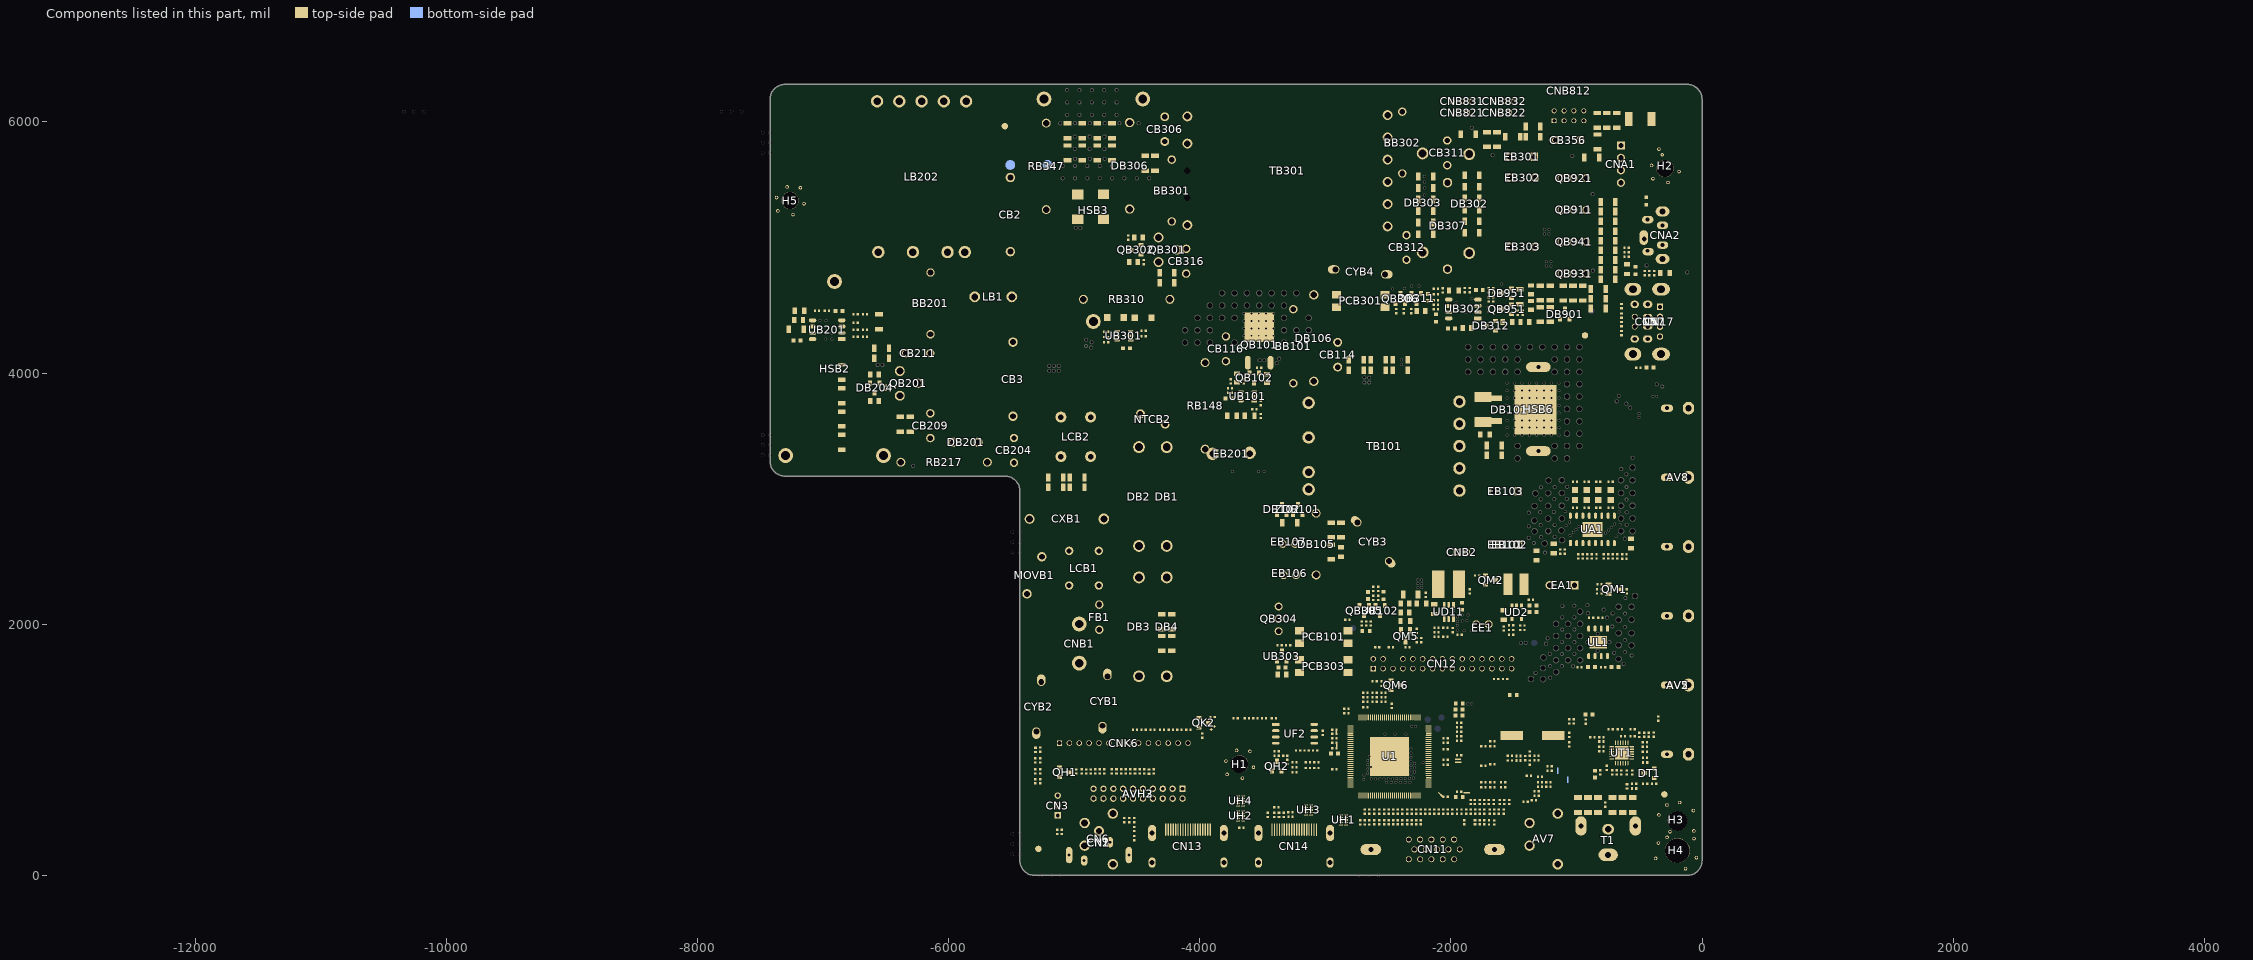
[diagram p0: the components of this part, seen from the top]
# Altium PCB MISC84277.PcbDoc (part 5 of 15)
Units mil, origin at the board's own origin, x right, y up, seen from the top; angles counter-clockwise.
Board outline 7422.08 x 6299.21 mil, 2 copper layers (TopLayer, BottomLayer), stack 61.855 mil thick; 709 components, 395 nets, 2812 pads, 811 vias.

## Footprints (in the part's own frame and the unit in brackets; to place one, negate y for a bottom-side part, rotate by r counter-clockwise, add the part's x,y. Pads: shape width x height; smd on the part's side, far side on the other; paste and mask are expansions set on the pad) (continued)
USB2-HD-1 [mm] "双盟 DUAL USB A/F 90°"
  oval 2.9x3.7 on Top Overlay: 0(-6.57,16) 0(-6.57,10.3) 0(6.57,16) 0(6.57,10.3)
  round 1.85 on Top Overlay: 0(-3.5,13.01) 0(-3.5,15.63) 0(3.5,13.01) 0(3.5,15.63)
  round 1.4 on Top Overlay: 0(-1,15.63) 0(-1,13.01) 0(1,15.63) 0(1,13.01)
  oval 1.5x1.7 hole 0.9: 1(-3.5,15.63) 4(3.5,15.63) 5(-3.5,13.01) 8(3.5,13.01)
  round 1.2 hole 0.9: 2(-1,15.63) 3(1,15.63) 6(-1,13.01) 7(1,13.01)
  oval 2.6x3.4 hole 1.6 slot 2.3 at 90 deg: 9(-6.57,16) 10(6.57,16) 11(-6.57,10.3) 12(6.57,10.3)
  KeepOutLayer pour cut-out: -5.206,13.033 -5.206,15.649 -4.578,15.021 -4.578,13.669 -5.214,13.033
  KeepOutLayer pour cut-out: -3.49,14.749 -4.146,14.618 -4.703,14.246 -5.075,13.69 -5.206,13.033 -5.206,13.033 -5.206,12.993 -5.068,12.303 -4.677,11.718 -4.092,11.327 -3.402,11.19 -3.402,11.19 2.42,11.19 2.637,11.233 2.821,11.356 2.943,11.539 2.986,11.756 2.986,11.756 2.986,14.202 2.944,14.414 2.824,14.594 2.644,14.714 2.432,14.756 2.432,14.756 -3.482,14.756 -3.485,14.756 -3.487,14.754 -3.489,14.752 -3.49,14.749
  KeepOutLayer pour cut-out: -3.49,17.369 -4.146,17.238 -4.703,16.866 -5.075,16.31 -5.206,15.653 -5.206,15.653 -5.206,15.613 -5.068,14.923 -4.677,14.338 -4.092,13.947 -3.402,13.81 -3.402,13.81 2.42,13.81 2.637,13.853 2.821,13.976 2.943,14.159 2.986,14.376 2.986,14.376 2.986,16.822 2.944,17.034 2.824,17.214 2.644,17.334 2.432,17.376 2.432,17.376 -3.482,17.376 -3.485,17.376 -3.487,17.374 -3.489,17.372 -3.49,17.369
  silkscreen extent -6.7,2 6.7,17.25, body extent -7.5,0 7.5,17, height 16.1
VR(13*5)-V-7.5 [mm] "TVR10561KSW(为勤)"
  round 1.9 hole 1.2: 1(3.75,-1.5) 2(-3.75,1.5)
  round 2.1 on Top Overlay: 2(-3.75,1.5) 2(3.75,-1.5)
  silkscreen extent -6.65,-2.5 6.42,2.5
XTAL-S-1 [mm] "假贴晶振（威特电子）"
  rect 4.6x1.8 smd: 1(-4.207,0) 2(4.207,0)
  silkscreen extent -5.8,-2.41 5.8,2.41, body extent -6.4,-2.36 6.39,2.38, height 5

## Part data
AV2 AV8: library part "RCA端子,RCA Jack,AV3,H,Yellow、White、Red,CH5.5,D14,Seal,DIP,RC075-F03L3BY-A,YUQIU-DLMI-AV", "CN-AV-D14-#-#"
AV5: library part "RCA端子,RCA Jack,AV3,H,Green、Blue、Red,CH5.5,D14,Seal,DIP,RC075-F03L3BY-B,YUQIU-DLMI-YPbPr", "CN-YPbPr-D14-#-#"
AV7: library part "耳机端子,Earphone  Jack,H,Φ3.5,CH7.0,Black,Seal,SMD,PJ7723-F03L3BE-C,YUQIU-DLMI", "CN-headphone"
AVH2: library part "连接插座,connect jack,2×10Pin,D2.0,D,SNAP,Fool-proofing,Beige,L=2.6mm,DIP,CJ-DHMI", "CN-latched"
AVH3: library part 2*10PIN-2.0-D-H-M-DHMI, "CN-straight gold pin"
BB101: library part φ3.5×6.0×0.65mm-CP(编带/秀益达)-9-DAI, "Through-hole ferrite bead"
BB201: library part Φ3.5×9.0×0.65mm(编带/秀益达)-DLAI, "Through-hole ferrite bead"
BB301: library part φ3.5×6.0×0.65mm-CP(编带/秀益达)-DAI, "Through-hole ferrite bead"
BB302: library part φ3.5×6.0×0.65mm-CP(编带/RY)-DLAI, "Through-hole ferrite bead"
C1: library part 10uF-1206-X5R-±10%-16V-D
CA9 CA10 CA16 CA17 CA24 CA25 CB103 CB323 CB324 CF29 CF30 CF33: library part 1000pF-0402-X7R-±10%-50V-D
CA11 CA23 CD2 CD3 CD6 CL2 CL3 CL42 CL43: library part 0.1uF-0402-X5R-±20%-16V-D
CA12 CA13 CA14 CA18 CA19 CA20 CA21 CA22: library part 0.22uF-0402-X5R-±10%-16V-D
CA15: library part 1uF-0402-X5R-±20%-16V-D
CA31 CA32 CD13: library part 3300pF-0402-X7R-±10%-50V-D
CA40 CA41 CD1 CD5 CD8 CD9 CD10 CM5: library part 10uF-0805-X5R-±20%-16V-D
CA60 CA61 CT12 CT19: library part 0.022uF-0402-X7R-±10%-16V-D
CB2 CB3: library part MPX450K474(散装/日精)-DHMI, "CAP(474)"
CB101 CB303 CB305 CI2 CO9 CT17: library part 100pF-0402-NPO-±5%-50V-D
CB102 CB109 CB206 CB304 CB321: library part 0.1uF-0603-X7R-±10%-50V-D, "CAP"
CB110 CB340: library part 1000pF-0402-X7R-±10%-50V-D, "CAP"
CB111 CB112: library part 1uF-0805-X7R-±10%-25V-D, "CAP"
CB113: library part 220PF-0805-NPO-±10%-200V-D, "CAP"
CB114 CB306: library part C242G472J20A201(编带/法拉)-DAI, "CAP"
CB116 CB209 CB316: library part "陶瓷电容,CAP CD,1KV,100pF,±10%,SL,P,5.0mm,DIP,TP,SHM-DHAI", "CAP"
CB118: library part 1000pF-0805-NPO-±10%-200V-D, "CAP"
CB201: library part 0.047uF-0603-X7R-±10%-25V-D
CB204: library part "陶瓷电容,CAP CD,1KV,4700pF,±20%,Y5U,P,5.0mm,DIP,TP,SHM-DHAI"
CB205: library part 220pF-0402-NPO-±5%-50V-D
CB211 CB312: library part CC45SL3AD470JYPNA(TDK)-DHAI, "CAP"
CB212: library part 0.22uF-0805-X7R-±10%-50V-D
CB221 CB301 CO10 CO11: library part 4700pF-0402-X7R-±10%-50V-D
CB302: library part "陶瓷电容,CAP MC,25V,1uF,±10%,X7R,0603,SMD,TP-D", "CAP"
CB311: library part "CAP CD,1KV,1000pF,±10%,Y5R,P,5.0mm,DIP,TP,SHM-DHAI", "CAP"
CB322: library part 0.022uF-0603-X7R-±10%-25V-D
CB326: library part 0.33uF-0805-X7R-±10%-50V-D, "C"
CB327 CB951: library part 0.1uF-0402-X7R-±10%-16V-D, "CAP"
CB328: library part 0.047uF-0805-X7R-±10%-50V-D
CB350: library part 0.47uF-0603-X5R-±10%-16V-D
CB356: library part CK45-B3AD102KYPNX(TDK)-DHAI, "CAP"
CD4 CD11 CD14 CD15 CF3 CF5 CF15 CF22 CF28 CF37 CL4 CL44 CT2 CT6 CU1: library part 10uF-0603-X5R-±20%-6.3V-D
CD7 CI8 CK6 CO8: library part 10pF-0402-NPO-±5%-50V-D
CD12 CD16 CD17 CF2 CF7 CF8 CF9 CF10 CF12 CF13 CF14 CF17 CF27 CG1 CG2 CH4 CH8 CH9 CH15 CI3 CI4 CI5 CI6 CK1 CK3 CK10 CM1 CM2 CM4 CO6 CT1 CT5 CT9 CT11 CT18 CT20 CT21 CT23 CT25 CT27 CT30 CV5 CV6: library part 0.1uF-0402-Y5V-+80%-20%-16V-D
CF1 CF32 CF38 CF39: library part 30pF-0402-NPO-±5%-50V-D
CF4 CH3 CH7 CH10 CT7 CT8 CV9 CV10: library part 33pF-0402-NPO-±5%-50V-D
CF6 CF11 CF16 CF18 CF19 CF20 CF21 CF23 CF24 CF25 CO1 CO4: library part 1uF-0402-X5R-±20%-6.3V-D
CF26 CF31 CF34 CI1 CI7 CI9 CI11 CV1 CV3 CV7: library part 0.047uF-0402-X7R-±10%-16V-D
CF35 CF36: library part 5pF-0402-NPO-±5%-50V-D
CK2 CM7: library part 0.01uF-0402-X7R-±10%-50V-D
CM3: library part 0.22uF-0402-Y5V-+80%-20%-16V-D
CN1: library part "RCA端子,RCA Jack,AV1,H,Yellow,CH5.5,Seal,DIP,AV38A-01S-5030,QS-DLMI"
CN2: library part "RCA端子,RCA Jack,AV1,H,Orange,CH5.5,Seal,DIP,AV38A-01S-5020,QS-DLMI"
CN3: library part 3PIN-2.0-D-H-G-DHMI
CN5: library part USB-A/F-90°-DLMI-USB, "CN-USB-double-deck-#-#"
CN6: library part "耳机端子,Earphone  Jack,H,Φ3.5,CH7.0,Black,switch,Seal,SMD,PJ7724-F05L3BE-D,YUQIU-DLMI-headphone", "CN-headphone-#-#-#"
CN7: library part USB-2035A01-DHMI-USB, "CN-USB-#-#-#"
CN11: library part WLHD-051A-DLMI-DB15, "CN-DB15-horizontal-#-#-#"
CN12: library part 2×15PIN-2.0-D-H-M(脚长=2.6mm)(缺6PIN)-LD-DHMI, "CN-straight gold pin"
CN13 CN14: library part 161031041(外壳SPCC)-D, "CN-HDMI-horizontal-#-#"
CN17: library part 4PIN-2.0-D-H-G-DHMI
CNA1: library part 4PIN-2.54-D-H-G-DHMI
CNA2: library part PJ-339-DLMI-headphone, "CN-headphone-#-#-#"
CNB1: library part "连接插座,connect jack,2Pin,D7.92,L,SNAP,Fool-proofing,nature,L=2.8mm,DIP,AMA-DLMI", "AC socket"
CNB2: library part 2PIN-2.0-D-H-G-B-DHMI, "Socket"
CNB812: library part 2×4PIN-2.0-L-H-F-镀金-LK-DLMI, "CN-gold pin"
CNB821 CNB822: library part 2PIN-2.0-D-H-G-DHMI
CNB831 CNB832: library part 3PIN-2.0-D-H-G-DHMI, "Socket"
CNK6: library part 14PIN-2.0-D-H-G-DHMI
CO7: library part 330pF-0402-X7R-±10%-50V-D
CT10 CT24: library part 56pF-0402-NPO-±5%-50V-D
CT13: library part 1.8pF-0402-NPO-±0.25pF-50V-D
CT26: library part 330pF-0402-NPO-±5%-50V-D
CT29: library part 6800pF-0402-X7R-±10%-50V-D
CT40: library part 470pF-0402-X7R-±10%-50V-D
CT41 CT42 CT43 CT44 CT45 CT46: library part 1000pF-1206-X7R-±20%-2000V-D
CXB1: library part "X电容,CAP X2,MP,275VAC,0.47uF,±10%,S,15mm-Mini,PC,DIP,BM-DHMI", "CAP"
CYB1 CYB2: library part CD70-B2GA221KYPKA(S/TDK)-DHMI, "CAP"
CYB3 CYB4: library part CD70ZU2GA102MYPKA(S/TDK)-DHMI, "CAP"
DB1 DB2 DB3 DB4: library part 1N5408G(编带/GOOD-ARK)-DLMI, "Diode"
DB101: library part MBRB10150CT(GOOD-ARK)-D, "Diode"
DB102 DB204: library part LBAV70LT1G(LRC)-D, "Diode"
DB105: library part 1N4007-DO-41-DLAI, "Diode"
DB106 DB306 DB307: library part FR207(编带/LRC)-DLAI, "Diode"
DB201: library part "整流二极管,DIO FRD S,8A,600V,ITO-220AC,DIP,UGF8J C0G,TSC-DHMI", "Diode"
DB202 DB203: library part GS3J-B(GULF)-D, "Diode"
DB302 DB303: library part "整流二极管,DIO FRD S,4A,800V,DO-201AD,DIP,MUR480-84mil,GOOD-ARK-DLMI", "Diode"
DB310 DB370 DB371: library part M7(WEJ)-D, "Diode"
DB311 DB901 DB951: library part LBAV70LT1G(LRC)-D
DB312: library part BAW56(NXP)-D
DH1 DH2 DH3 DH4 DH5 DH6 DH7 DH8 DH9 DH10 DK1: library part AVLC18S02003-D
DT1: library part BAV99-BR-D
DU1 DU3 DU4 DU7 DU8: library part AIES12U020R2-D
EA1: library part 470uF-16V±20%-10×12-105℃-编带-F=5.0-XL-DHAI
EB101 EB103: library part 470uF-25V-±20%-10×12.5-105℃-GF-编带-F=5.0(CapXon)-DHAI, "Electrolytic"
EB102: library part 270uF-16V-±20%-8×11.5-105℃-PS-短脚-F=3.5(Capxon), "Solid-state"
EB106: library part 100uF-35V-±20%-6.3×11-105℃-KF-编带-F=2.5(CapXon)-DHAI, "Electrolytic"
EB107: library part 10uF-50V-±20%-5×11-105℃-GH-编带-F=2.5(CapXon)-DHAI, "Electrolytic"
EB201: library part 100uF-450V-±20%-16×35.5-105℃-KM-折脚(H=8.1mm)(Capxon)-DLMI, "Electrolytic"
EB301: library part 68uF-160V-±20%-12.5×20-105℃-RR-编带-F=5.0(Samxon)-DHMI, "Electrolytic"
EB302 EB303: library part "铝电解电容,CAP AL,200V,33uF,±20%,LD,KF,P,5.0mm,13×13,DIP,TP,CapXon-DHAI", "Electrolytic"
EE1: library part 470uF-10V-±20%-6.3×11-105℃-黑底白字-编带-F=2.5-XF-DHAI, "Electrolytic"
EVA1 EVA2 EVA3 EVA4 EVA5 EVA6 EVA7: library part 7×7×3mm-C-4305防火泡棉-黑色-DLMI, "EVA"
F2 RU1 RU2 RU3 RU4: library part 5R1ohm-0402-±5%-1/16W-D
FB1: library part 2010T3.15A250VA1(编带/华德)-DHAI, "FUSE"
GD1 GD2 GD3 GD4: library part 7.00×8.54mm-尼龙-白色-DHMI
GL1 GL2 GL3 GL4: library part SLD-8854W-白胶, "White glue"
H1 H2 H3 H4 H5: library part "Location hole-D"
HS: library part TEST
HSB2: library part 40×25×5.0-黑色-带引脚(厚=1.5mm)-FR-DLMI, "Heatsink"
HSB3: library part 50×25×5.0-黑色-带引脚(厚=1.5mm)-FR-DLMI, "Heatsink"
HSB6: library part 17.5×14.5×0.5-本色-Cu-MRD-D, "Heatsink"
JB102 JB103 JB106 JB107 RB904 RB905: library part 0ohm-1206-±5%-1/4W-D, "RES"
LB1: library part SYDR1212-L003-EDL-DHMI, "I-shaped inductor"
LB202: library part SYEQ2612-L250uA-SQ-DLMI, "PFC inductor"
LBA1 LBA2 LBA3 LBA4: library part 300ohm-2500mA-0805-D
LCB1: library part SYT10-L002-SQ-DHMI, "Common mode"
LCB2: library part SYT14-L003-JM-DLMI, "Common mode"
LD2: library part CTD0403-6R8-M-D
LD12: library part CTD0504-4R7-M-D
LF1 LF2 LF3 LF4 LF5 LF6 RA7 RA11: library part GND
LF7: library part SDCL1005CR33JTDF-D
LT1: library part SDCL1005C68NJTDF(68nH-0402±5%-C)-D
LT2 LT6 LT8 RT1 RT14: library part 1Kohm-0402-±25%-D
LT3: library part 2.2nH-0402-±0.3nH-1/4-D
LT9 LT11: library part SDCL1005CR27JTDF(顺络)-D
LT10: library part SDCL1608CR22JT(F)-D
M1 M2 M3 M4: library part MARK-D
MB1 MB2: library part PM3.0×8.0×5.5mm-银色-双垫片-DHMI, "SCREW"
ML1: library part MALAY
MOVB1: library part TVR10561KSC3AGGW(短脚/为勤)-DHMI, "Varistor"
NTCB2: library part SCK102R55AMBY502(短脚/为勤)-DHMI, "Thermistor"
PCB101: library part LTV-817S-TA-B(光宝)-DMI, "Optocoupler"
PCB301 PCB303: library part LTV-817S-TA-B(光宝)-D, "Optocoupler"
QB101: library part 场效应管,NMOS,5A,700V,0.9ohm@ID=2.5A@VGS=10V,TO-252,MMD70R900PRH,MAGNACHIP-D, "N Channel Single MOSFET"
QB102 QB302 QB306: library part 3CG3906M-D, "Transistor"
QB201: library part TK15A50D(东芝)-DLMI, "MOS"
QB201和散热片之间 QB301和散热片之间: library part 0.05g-导热硅脂, "Thermal grease"
QB301: library part MDF7N65BTH(Magnachip)-DLMI, "MOS"
QB304: library part 2N4401(蓝箭)-DAI
QB305 QB951 QM2 QM6: library part LMBT3904LT1G-D-NPN, "Q-NPN-#-#-#"
QB911 QB921 QB931 QB941: library part 2SD1857L-Q-T9N-B(UTC)-DAI, "Transistor"
QH1 QH2 QK2: library part MMBT3904(f≥350MHz)-D-NPN, "Q-NPN-#-#-#"
QM1: library part WPM2341A-3/TR-D
QM5: library part WPM3407C-3/TR-D
R1 R2 R3 R4 RB143 RD13 RG2 RI1 RI2 RK10 RO2 RO6 RO13 RO15 RO16 RO17 RT7: library part 0ohm-0402-±5%-1/16W-D
R5V R12V: library part 0ohm-0805-±5%-1/8W-D
RA1 RA8 RF10 RF11 RH19 RH20 RM8 RO10 RT2 RV10 RV12: library part 100ohm-0402-±5%-1/16W-D
RA4 RA12 RA28 RB221 RH5 RH14 RK2 RK3 RK16 RK21: library part 1Kohm-0402-±5%-1/16W-D
RA9 RA14: library part 330ohm-0402-±5%-1/16W-D
RA10 RA17: library part 0ohm-0603-±5%-1/10W-D
RA23: library part 1kohm-0402-±5%-1/16W-D
RB1 RB2 RB3 RB4: library part 1M2ohm-1206-±5%-1/4W-D, "RES"
RB101 RB102: library part 330Kohm-1206-±5%-1/4W-D, "RES"
RB103 RK8: library part 10Kohm-0402-±1%-1/16W-D
RB104 RB226 RB366: library part 47Kohm-0402-±1%-1/16W-D
RB105 RB107 RB215 RB305 RB307 RB346 RG1 RO1 RO5: library part 510ohm-0402-±5%-1/16W-D
RB106 RB365: library part 68ohm-0805-±5%-1/8W-D
RB108 RB213 RB308: library part 20ohm-0805-±5%-1/8W-D, "RES"
RB109 RB214 RB225 RB309: library part 10Kohm-0402-±5%-1/16W-D, "RES"
RB110 RB114 RB115 RB116 RB117 RB118 RB210 RB314 RB315 RB911 RB912 RB913 RB921 RB922 RB923 RB931 RB932 RB933 RB941 RB942 RB943: library part 10ohm-1206-±5%-1/4W-D, "RES"
RB123 RB124: library part 47ohm-1206-±5%-1/4W-D, "RES"
RB131: library part 2Kohm-0603-±5%-1/10W-D
RB132 RB133: library part 3Kohm-0402-±5%-1/16W-D, "RES"
RB134: library part 4K7ohm-0402-±1%-1/16W-D, "RES"
RB135: library part 18Kohm-0402-±1%-1/16W-D, "RES"
RB141 RB142: library part 2Mohm-1206-±5%-1/4W-D, "RES"
RB144 RB145 RB146 RB147 RB317 RB318 RB319 RB320 RB321 RB322 RB323 RB324: library part 100Kohm-1206-±5%-1/4W-D, "RES"
RB148 RB310: library part MOF-0R27ohm-±5%-2WS(编带/Futaba)-DLAI, "RES"
RB201 RB202 RB203 RB204: library part 1Mohm-1206-±1%-1/4W-D, "RES"
RB205: library part 560kohm-0402-±1%-1/16W-D
RB206 RB349: library part 27Kohm-0402-±1%-1/16W-D, "RES"
RB209: library part 39Kohm-0805-±1%-1/8W-D, "RES"
RB212 RB301 RB306: library part 47ohm-0805-±5%-1/8W-D, "RES"
RB217: library part MOF-0R1ohm-±5%-2WS(编带/Futaba)-DLAI, "RES"
RB218: library part 1R6ohm-1206-±1%-1/4W-D, "RES"
RB219 RB220: library part 100ohm-1206-±5%-1/4W-D, "RES"
RB223 RB224 RB391 RB392: library part 22ohm-1206-±5%-1/4W-D
RB227: library part 0ohm-0402-±5%-1/16W-D, "RES"
RB302: library part 8K2ohm-0402-±1%-1/16W-D
RB303 RB351 RF2 RH1 RH2 RH3 RH4 RH6 RH7 RH8 RH9 RH10 RH11 RH15 RH16 RI4 RI6 RI8 RI10 RK20 RM3 RM4 RT18 RV6 RV7 RV13 RV14: library part 10Kohm-0402-±5%-1/16W-D
RB304 RD8 RO3 RO7: library part 47Kohm-0402-±5%-1/16W-D
RB325: library part 49K9ohm-0402-±1%-1/16W-D
RB326: library part 1Kohm-0805-±5%-1/8W-D, "R"
RB328 RB329 RB330 RB331 RB332 RB334 RB335: library part 270Kohm-1206-±5%-1/4W-D
RB333: library part 200Kohm-1206-±5%-1/4W-D, "RES"
RB337 RB339 RB340: library part 4R7ohm-1206-±1%-1/4W-D, "RES"
RB338: library part 8R2ohm-1206-±5%-1/4W-D, "RES"
RB341: library part 2R2ohm-1206-±1%-1/4W-D, "RES"
RB345: library part 5K6ohm-0402-±1%-1/16W-D, "RES"
RB347: library part MOF-300Kohm-±5%-2WS(编带/Futaba)-DLAI, "RES"
RB348 RB367: library part 1Kohm-0402-±5%-1/16W-D, "RES"
RB350 RB384: library part 1Kohm-0603-±1%-1/10W-D
RB352: library part 20Kohm-0402-±1%-1/16W-D, "RES"
RB354: library part 2Kohm-0402-±1%-1/16W-D, "RES"
RB355: library part 3K9ohm-0402-±1%-1/16W-D
RB356: library part 2M2ohm-0402-±5%-1/16W-D
RB357: library part 3Kohm-0402-±1%-1/16W-D
RB358 RB359: library part 150Kohm-0805-±1%-1/8W-D, "RES"
RB360 RB361 RB362 RB363: library part 150Kohm-1206-±5%-1/4W-D, "RES"
RB364: library part 30Kohm-0805-±1%-1/8W-D
RB368 RB369 RB370 RB371: library part 68ohm-1206-±5%-1/4W-D, "RES"
RB385 RK4: library part 4K7ohm-0402-±1%-1/16W-D
RB386: library part 9K1ohm-0402-±1%-1/16W-D
RB901 RB902 RB903: library part 470ohm-1206-±5%-1/4W-D, "RES"
RB951: library part 2Kohm-0402-±1%-1/16W-D
RB952: library part 20Kohm-1206-±5%-1/4W-D
RD1 RM2: library part 100Kohm-0402-±5%-1/16W-D
RD6: library part 12Kohm-0402-±1%-1/16W-D
RD7: library part 12K4ohm-0402-±1%-1/16W-D
RD12: library part 30Kohm-0402-±1%-1/16W-D
RD15 RK1: library part 22ohm-0402-±5%-1/16W-D
RD16 RK7: library part 5K6ohm-0402-±1%-1/16W-D
RF1: library part 1Mohm-0402-±5%-1/16W-D
RF3 RF8 RF9 RF13 RF18 RK15 RK18 RT3 RT4: library part 4K7ohm-0402-±5%-1/16W-D
RF12 RF16 RF19: library part 68ohm-0402-±5%-1/16W-D
RF14 RF15 RM7: library part 200Kohm-0402-±5%-1/16W-D
RH13 RO9 RT9 RT10: library part 220ohm-0402-±5%-1/16W-D
RH55: library part 33Kohm-0402-±5%-1/16W-D
RH56: library part 22Kohm-0402-±5%-1/16W-D
RI3: library part 150ohm-0402-±5%-1/16W-D
RI5 RI7 RI9 RI11 RV4 RV8: library part 12Kohm-0402-±5%-1/16W-D
RI12 RI14 RI16 RT5 RT6 RV1 RV3 RV9: library part 33ohm-0402-±5%-1/16W-D
RI13 RI15 RI17 RI18 RO12 RV2 RV5 RV11: library part 75ohm-0402-±5%-1/16W-D
RK5 RM10: library part 2K2ohm-0402-±5%-1/16W-D
RK6: library part 680ohm-0402-±5%-1/16W-D
RK9: library part 20Kohm-0402-±1%-1/16W-D
RK11: library part 1K2ohm-0402-±5%-1/16W-D
RM1 RM5 RM6: library part 4k7ohm-0402-±5%-1/16W-D
RT11: library part 1K8ohm-0402-±5%-1/16W-D
RT12: library part 820ohm-0402-±5%-1/16W-D
T1: library part RF-A814.5(H=6.3mm)-DLMI, "T-IEC-6.3mm-#-#"
TB101: library part SYEQ2612-T012A-YX-DLMI, "Transformer"
TB301: library part SYEFD30-T009-XX-DLMI, "Transformer"
TP-TDT: library part TEST, "TEST"
U1: library part TSU69ZR-D
UA1: library part "音频功放,IC Audio AMP,Class D,2×13W@13.0V@8ohm,TSSOP16,SMD,OB6223BPA,On-bright-D"
UB101 UB301: library part "LD5530 RGL(通嘉)-D", "IC"
UB102 UB303: library part AZ431AN-ATRE1(BCD)-D, "SMD 431"
UB201: library part "PWM控制器,IC PWM Controller,300KHz,SOP-8,SMD,FAN7930CMX_G,Fairchild-D", "IC"
UB302: library part "运算放大器,IC AMP,2 channel,SOIC8,SMD,BA10358F-BZSE2,ROHM-D", "Operational Amplifier"
UD2: library part LC3406CB5TR-D
UD11: library part RT6212
UF2: library part "SPI FLASH оƬ,IC SPI FLASH,32Mb,SOIC8,SMD,GD25Q32CSIG,GigaDevice-D"
UH1 UH2 UH3 UH4: library part ULC0524P-D, "RCLAMP0524J"
UL1: library part LC1118-D
UT1: library part R840-D
YF1: library part 24MHz-±20PPM-20PF-HC-49S-SMD-D
ZDB101: library part BZX84C24(蓝箭)-D, "Diode"
硅胶: library part Φ12mm×12mm-黑色-125度(UL认证)-D